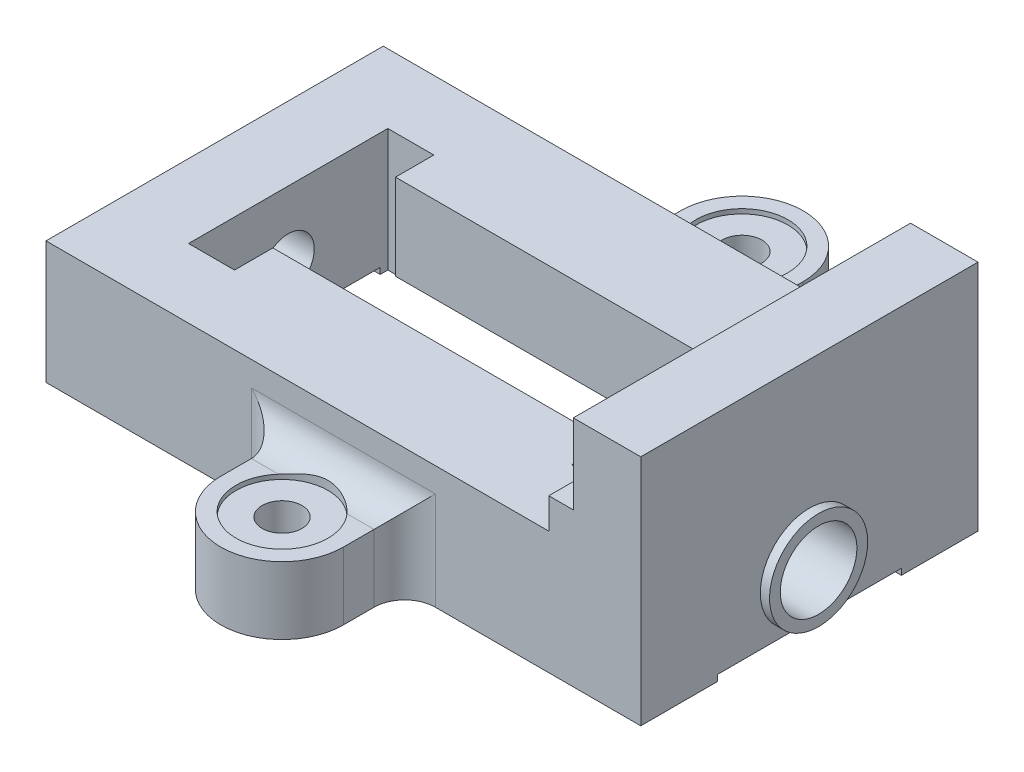
SolidWorks part; units mm, degrees
ref_plane "Front Plane" through (0, 0, 0) normal (0, 0, 1) x (1, 0, 0)
ref_plane "Top Plane" through (0, 0, 0) normal (0, 1, 0) x (1, 0, 0)
ref_plane "Right Plane" through (0, 0, 0) normal (1, 0, 0) x (0, 0, -1)
sketch "Sketch1" plane through (0, 0, 0) normal (0, 0, 1) x (1, 0, 0)
  line L0 (0, 0) -> (194, 0)
  line L1 (194, 0) -> (194, 29.3329)
  line L3 (194, 29.3329) -> (194, 76)
  line L4 (194, 76) -> (172, 76)
  line L5 (172, 76) -> (172, 50)
  line L6 (172, 50) -> (164, 50)
  line L7 (164, 50) -> (164, 40)
  line L8 (164, 40) -> (0, 40)
  line L9 (0, 40) -> (0, 0)
  dimension "D1" = 76
  dimension "D2" = 194
  dimension "D3" = 26
  dimension "D4" = 8
  dimension "D5" = 22
  dimension "D6" = 40
extrude "Boss-Extrude1" add sketch "Sketch1" along normal mid plane 110
sketch "Sketch2" plane through (194, 0, 0) normal (1, 0, 0) x (0, 0, -1)
  line L0 (-55, 0) -> (55, 0) construction
  line L1 (-30, 0) -> (30, 0)
  line L2 (-30, 0) -> (-30, 2)
  line L3 (-30, 2) -> (30, 2)
  line L4 (30, 0) -> (30, 2)
  point P6 (0, 2)
  dimension "D1" = 60
  dimension "D2" = 2
extrude "Cut-Extrude1" cut sketch "Sketch2" against normal blind 212
sketch "Sketch3" plane through (194, 0, 0) normal (1, 0, 0) x (0, 0, -1)
  circle A0 centre (0, 18) radius 16
  dimension "D2" = 32
  dimension "D1" = 18
extrude "Boss-Extrude2" add sketch "Sketch3" along normal blind 3
sketch "Sketch4" plane through (197, 0, 0) normal (1, 0, 0) x (0, 0, -1)
  circle A0 centre (0, 18) radius 12.5
  dimension "D1" = 25
extrude "Cut-Extrude2" cut sketch "Sketch4" against normal blind 56
sketch "Sketch5" plane through (0, 0, 0) normal (-1, 0, 0) x (0, 0, 1)
  circle A0 centre (0, 18) radius 12.5
  dimension "D2" = 25
  dimension "D1" = 18
extrude "Boss-Extrude3" add sketch "Sketch5" along normal blind 3
sketch "Sketch6" plane through (-3, 0, 0) normal (-1, 0, 0) x (0, 0, 1)
  circle A0 centre (0, 18) radius 8.5
  dimension "D1" = 17
extrude "Cut-Extrude3" cut sketch "Sketch6" against normal blind 66
sketch "Sketch7" plane through (0, 40, 0) normal (0, 1, 0) x (1, 0, 0)
  line L0 (164, -55) -> (164, 55) construction
  line L1 (164, 32.5) -> (149, 32.5)
  line L2 (164, 32.5) -> (164, -32.5)
  line L3 (164, -32.5) -> (149, -32.5)
  line L4 (149, 32.5) -> (149, 20)
  line L5 (39, -20) -> (39, -32.5)
  line L6 (149, 20) -> (39, 20)
  line L8 (149, -20) -> (39, -20)
  line L10 (39, 32.5) -> (24, 32.5)
  line L11 (39, 32.5) -> (39, 20)
  line L12 (39, -32.5) -> (24, -32.5)
  line L13 (24, 32.5) -> (24, -32.5)
  line L14 (149, -20) -> (149, -32.5)
  point P9 (24, 0)
  point P18 (164, 0)
  dimension "D1" = 65
  dimension "D2" = 15
  dimension "D3" = 15
  dimension "D4" = 20
  dimension "D5" = 40
  dimension "D6" = 110
extrude "Cut-Extrude4" cut sketch "Sketch7" against normal blind 28
sketch "Sketch9" plane through (0, 0, 0) normal (0, -1, 0) x (1, 0, 0)
  line L0 (197, -16) -> (197, 16) construction
  line L2 (117, 75) -> (117, 65)
  line L3 (0, 55) -> (194, 55) construction
  line L4 (97, 75) -> (97, 40.778) construction
  line L5 (77, 75) -> (77, 65)
  line L6 (67, 55) -> (127, 55)
  arc A0 (117, 75) -> (77, 75) centre (97, 75) ccw
  circle A1 centre (97, 75) radius 6.5
  arc A2 (117, 65) -> (127, 55) centre (127, 65) ccw
  arc A3 (77, 65) -> (67, 55) centre (67, 65) cw
  dimension "D1" = 40
  dimension "D4" = 13
  dimension "D5" = 10
  dimension "D2" = 100
  dimension "D3" = 75
extrude "Boss-Extrude4" add sketch "Sketch9" against normal blind 22
fillet "Fillet1" radius 10 1 edges at (97, 22, 55)
sketch "Sketch10" plane through (0, 22, 0) normal (0, 1, 0) x (1, 0, 0)
  circle A0 centre (97, -75) radius 15
  dimension "D1" = 30
extrude "Cut-Extrude5" cut sketch "Sketch10" against normal blind 1.5 and the other way blind 15.5
mirror "Mirror17" about plane through (0, 0, 0) normal (0, 0, 1) of bodies 114
sketch "Sketch12" plane through (0, 0, 0) normal (0, -1, 0) x (1, 0, 0)
  line L0 (39, 20) -> (149, 20) construction
  line L1 (39, 20) -> (149, 20)
  line L2 (164, 32.5) -> (164, -32.5)
  line L3 (39, 32.5) -> (149, 32.5)
  line L4 (149, -32.5) -> (39, -32.5)
  line L18 (164, 32.5) -> (164, 55)
  line L19 (149, 32.5) -> (164, 32.5)
  line L20 (149, 20) -> (149, 32.5)
  line L21 (39, 20) -> (149, 20)
  line L22 (39, 32.5) -> (39, 20)
  line L23 (24, 32.5) -> (39, 32.5)
  line L24 (24, -32.5) -> (24, 32.5)
  line L25 (39, -32.5) -> (24, -32.5)
  line L26 (39, -20) -> (39, -32.5)
  line L27 (149, -20) -> (39, -20)
  line L28 (149, -32.5) -> (149, -20)
  line L29 (164, -32.5) -> (149, -32.5)
  line L30 (164, -55) -> (164, -32.5)
  line L31 (0, -55) -> (164, -55)
  line L32 (0, 55) -> (0, -55)
  line L33 (164, 55) -> (0, 55)
  line L35 (149, 32.5) -> (164, 32.5)
  line L36 (149, 20) -> (149, 32.5)
  line L37 (39, 20) -> (149, 20)
  line L38 (39, 32.5) -> (39, 20)
  line L39 (24, 32.5) -> (39, 32.5)
  line L40 (24, -32.5) -> (24, 32.5)
  line L41 (39, -32.5) -> (24, -32.5)
  line L42 (39, -20) -> (39, -32.5)
  line L43 (149, -20) -> (39, -20)
  line L44 (149, -32.5) -> (149, -20)
  line L45 (164, -32.5) -> (149, -32.5)
  line M18 (194, -30) -> (0, -30)
  dimension "D1" = 0
extrude "Cut-Extrude7" cut sketch "Sketch12" against normal blind 12 contours L44 L2 L35 L36 L1 L38 L39 L40 L42 L43 M18 | L3 L38 L1 L36 | L4 L44 L42 M18 | L44 L43 L42 M18 | L42 L40 L41 M18 | L45 L2 L44 M18
sketch "Sketch13" plane through (172, 0, 0) normal (-1, 0, 0) x (0, 0, 1)
  line L0 (55, 76) -> (-55, 76) construction
  line L1 (0, 0) -> (0, 76) construction
  circle A0 centre (38, 63) radius 3
  circle A1 centre (-38, 63) radius 3
  dimension "D1" = 6
  dimension "D2" = 38
  dimension "D3" = 13
extrude "Cut-Extrude8" cut sketch "Sketch13" against normal blind 10
